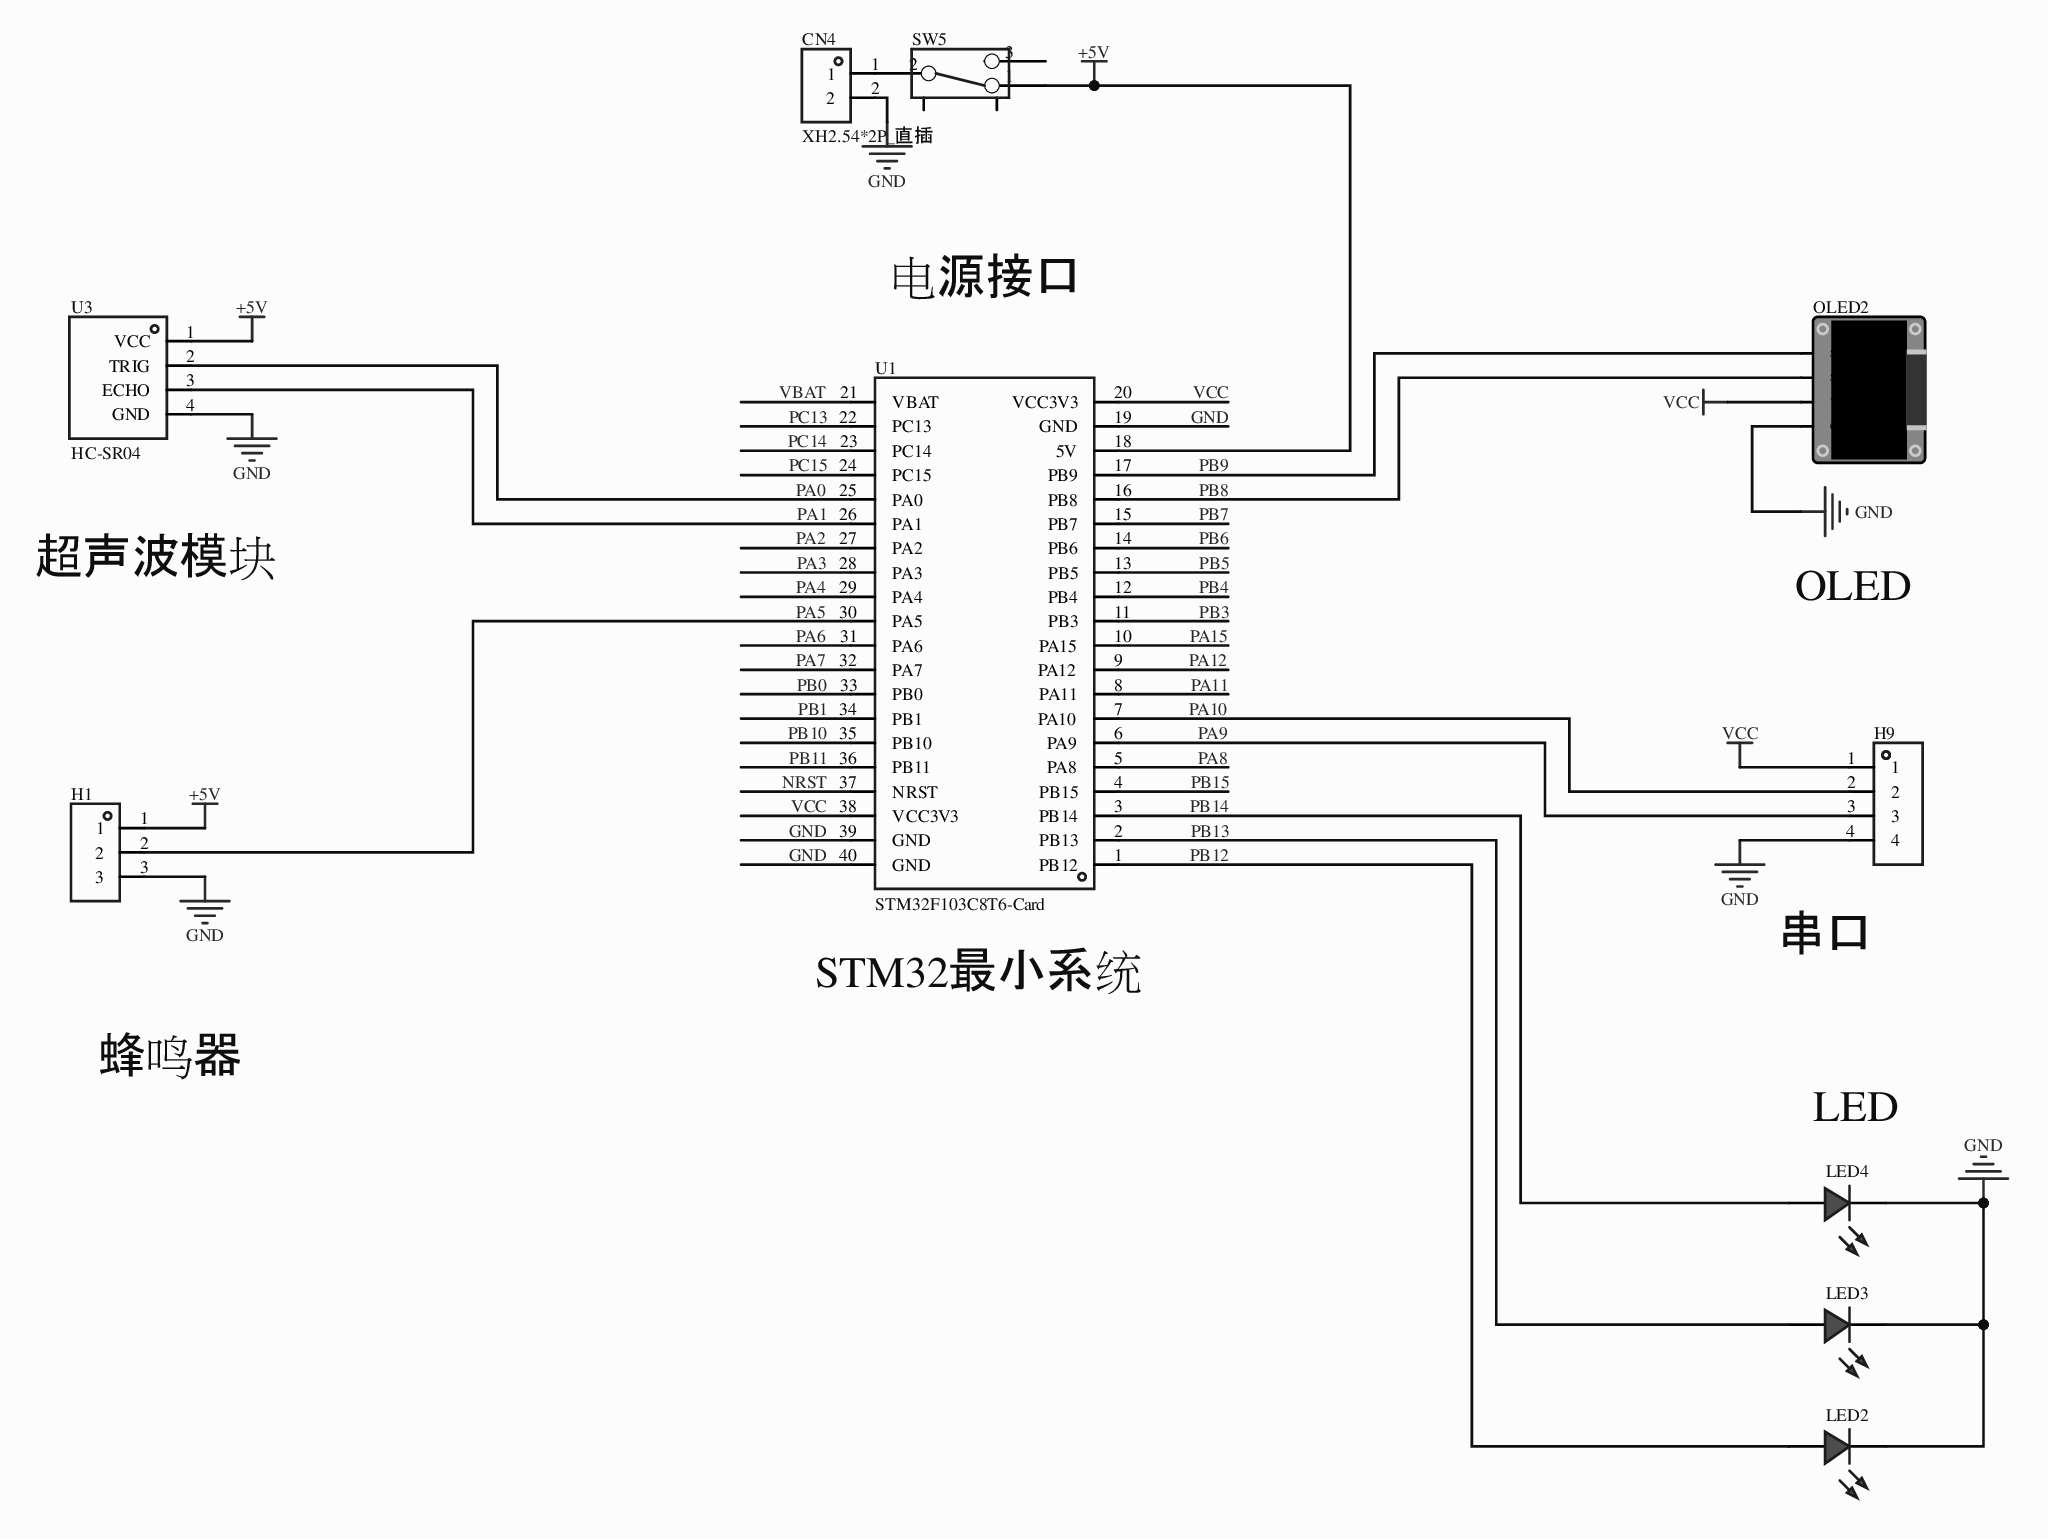
[diagram p0: MISC51194-3.schdoc]
# Altium project MISC51194-2.PrjPcb
1 sheet, 10 parts. Net scope: global (net labels, ports and power ports of the same name join across sheets).
Board file: MISC51194.pcbdoc

## Sheet MISC51194-3.schdoc
size 297 x 209 mm; Version: V1.0; @Project Name: MISC51194; @Page Count: 1; @Update Date: 2026-05-07; @Create Date: 2026-05-07; @Schematic Name: MISC51194; @Page No: 1; @Create Time: 23:22:16; @Update Time: 17:32:40; @Board Name: MISC51194

### Parts
CN4  XH2.54*2P_直插  [CONN-TH_2P-P2.50-XH2.54-2P]
H1  (no value)  [HDR-TH_3P-P2.54-V-F]
H9  (no value)  [HDR-TH_4P-P2.54-V-F]
LED2  (no value)  [LED_TH-3mm]
LED3  (no value)  [LED_TH-3mm]
LED4  (no value)  [LED_TH-3mm]
OLED2  (no value)  [0.96OLED_4P]
SW5  (no value)  [拨动开关]
U1  STM32F103C8T6-Card  [CONN-TH_L53.3-W22.9_STM32F103C8T6-CARD]
U3  HC-SR04  [TH_HC-SR04V]

### Nets
+5V: H1.1 SW5.1 U1.18(5V) U3.1(VCC)
GND: CN4.2 H1.3 H9.4 LED2.2(A) LED3.2(A) LED4.2(A) OLED2.1(GND) U1.19(GND) U1.39(GND) U1.40(GND) U3.4(GND)
VCC: H9.1 OLED2.2(VCC) U1.20(VCC3V3) U1.38(VCC3V3)
NRST: U1.37(NRST)
PA0: U1.25(PA0) U3.2(TRIG)
PA1: U1.26(PA1) U3.3(ECHO)
PA2: U1.27(PA2)
PA3: U1.28(PA3)
PA4: U1.29(PA4)
PA5: H1.2 U1.30(PA5)
PA6: U1.31(PA6)
PA7: U1.32(PA7)
PA8: U1.5(PA8)
PA9: H9.3 U1.6(PA9)
PA10: H9.2 U1.7(PA10)
PA11: U1.8(PA11)
PA12: U1.9(PA12)
PA15: U1.10(PA15)
PB0: U1.33(PB0)
PB1: U1.34(PB1)
PB3: U1.11(PB3)
PB4: U1.12(PB4)
PB5: U1.13(PB5)
PB6: U1.14(PB6)
PB7: U1.15(PB7)
PB8: OLED2.3(SCL) U1.16(PB8)
PB9: OLED2.4(SDA) U1.17(PB9)
PB10: U1.35(PB10)
PB11: U1.36(PB11)
PB12: LED2.1(C) U1.1(PB12)
PB13: LED3.1(C) U1.2(PB13)
PB14: LED4.1(C) U1.3(PB14)
PB15: U1.4(PB15)
PC13: U1.22(PC13)
PC14: U1.23(PC14)
PC15: U1.24(PC15)
VBAT: U1.21(VBAT)
NetCN4_1: CN4.1 SW5.2

Not connected (* = marked no-connect by the designer): SW5 3 4 5

### Notes on the sheet
- 电源接口
- 超声波模块
- OLED
- (near U1) STM32最小系统
- (near H9) 串口
- 蜂鸣器
- (near LED4) LED

### Library data of the parts
CN4 = XH2.54*2P_直插: 3D Model: 325c595e30db4df8abe76612dd40b0fa0819f05c4eef4c71ace90d822a990e87; 3D Model Transform: 295.275,228.346,0,180,0,0,-0.002,-20.079,-137.795; AddInBom: yes; Device: XH2.54*2P_直插; Symbol: XH2.54*2P_直插; LCSC Part Name: XH2.54*2P_直插; Supplier Part: C9900008615; Manufacturer Part: XH2.54*2P_直插; Supplier Footprint: XH2.54_2P; JLCPCB Part Class: Extended Part; Supplier: LCSC; FootprintName: CONN-TH_2P-P2.50-XH2.54-2P; ConvertToPcb: yes; ModelName: CONN-TH_2P-P2.50-XH2.54-2P
H1 = HDR-F_2.54_1x3P: Symbol: PM254V-11-03-H85; ConvertToPcb: yes; ModelId: f3b3cc5aae9641bf9e56fc160cef875b; ModelName: HDR2.54-F-LI-1X3P; ModelTransform: 299.9994,100,0,0,0,0,0,0,-118.11; Device: HDR-F_2.54_1x3P; AddInBom: yes; SupplierPart: C541850; Supplier Footprint: 插件; FootprintName: HDR-TH_3P-P2.54-V-F
H9 = HDR-F_2.54_1x4P: Symbol: 2.54-1*4P母; ConvertToPcb: yes; ModelId: d187812051054f85879fcaa51a310d8e0819f05c4eef4c71ace90d822a990e87; ModelTransform: 419.6842,98.464,0,0,0,0,0,0,-118.11; Device: HDR-F_2.54_1x4P; AddInBom: yes; SupplierPart: C2718488; Supplier Footprint: 插件; FootprintName: HDR-TH_4P-P2.54-V-F; ModelName: HDR-TH_4P-P2.54-V-F
LED2-LED4 = LED_TH-R_3mm: 3D Model: a497c992633541038a38947cdc58012f0819f05c4eef4c71ace90d822a990e87; 3D Model Transform: 141.274,153.327,0,0,0,0,-5.984,0,-137.795; ConvertToPcb: yes; ModelName: LED-TH-3mm_R; Symbol: LED_TH-R; Device: LED_TH-R_3mm; Supplier Footprint: 插件; AddInBom: yes; FootprintName: LED_TH-3mm
OLED2 = 0.96OLED模块_4P: 3D Model: 79c000fdb68d45a296c2e9bedf4f9055; 3D Model Transform: 1393.69792,1318.895,0,0,0,0,0,-560.079,-137.795; ConvertToPcb: yes; Symbol: 0.96OLED模块_4P; Device: 0.96OLED模块_4P; Supplier Footprint: 插件; AddInBom: yes; FootprintName: 0.96OLED_4P; ModelName: 0.96OLED_4P
SW5 = 拨动开关_正: ConvertToPcb: yes; ModelId: 4321fe59a4074cbfb4989553f297c68f0819f05c4eef4c71ace90d822a990e87; ModelName: SW-TH_SS-12D02-VG4; ModelTransform: 370.09,208.7,472.35,0,0,0,0,0,-110; Device: 拨动开关_正; Symbol: 拨动开关; FootprintName: 拨动开关; AddInBom: yes; Supplier Footprint: 插件
U1 = STM32F103C8T6-Card: AddInBom: yes; Device: STM32F103C8T6-Card; Symbol: STM32F103C8T6-CARD; FootprintName: CONN-TH_L53.3-W22.9_STM32F103C8T6-CARD; LCSC Part Name: STM32F103C8T6-Card; SupplierPart: C9900077949; ManufacturerPart: STM32F103C8T6-Card; Supplier Footprint: 插件; Supplier: LCSC; ConvertToPcb: yes
U3 = HC-SR04: Manufacturer: Universal Microelectronics; AddInBom: yes; Symbol: HC-SR04; Device: HC-SR04; LCSC Part Name: HC-SR04; SupplierPart: C19857336; ManufacturerPart: HC-SR04; Supplier Footprint: -; JLCPCB Part Class: 扩展库; Datasheet: https://atta.szlcsc.com/upload/public/pdf/source/20240122/47B8E374E428935B7962A2189EF91AAC.pdf; Supplier: LCSC; ConvertToPcb: yes; FootprintName: TH_HC-SR04V